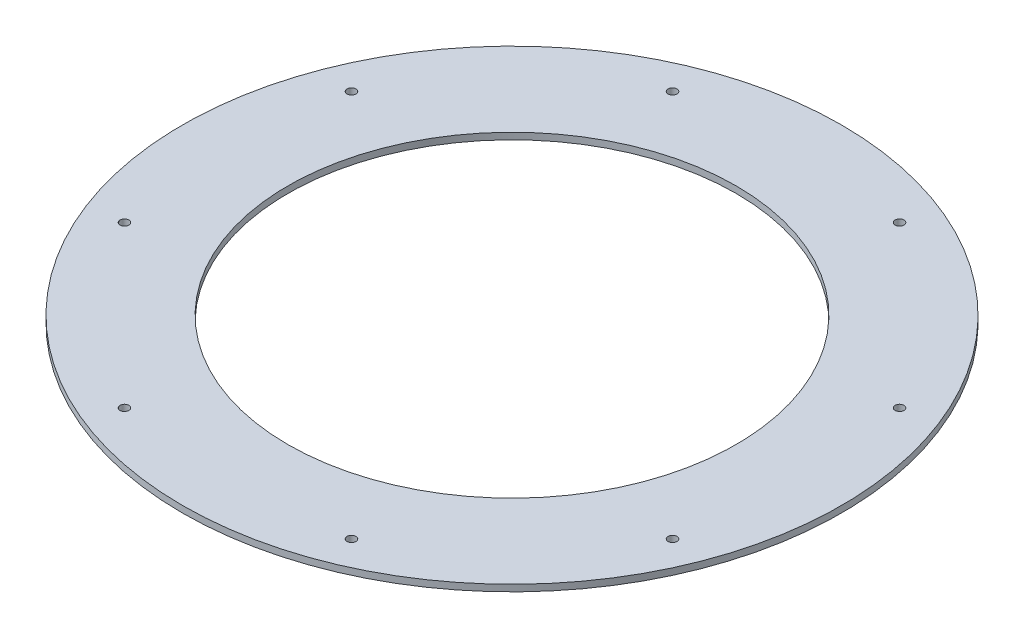
from build123d import *

# Parameters (mm, degrees)
SKETCH1_R                    = 500
SKETCH1_R_2                  = 340
BOSS_EXTRUDE1_DEPTH          = 5
F_13_5_13_5_DIAMETER_HOLE1_D = 13.5


with BuildPart() as part:
    # Sketch1 → Boss-Extrude1 (new, symmetric)
    with BuildSketch(Plane(origin=(0, 0, 0), x_dir=(1, 0, 0), z_dir=(0, 1, 0))):
        with Locations(Location((0, 0, 0), (0, 0, 270))):
            Circle(SKETCH1_R)
        with Locations(Location((0, 0, 0), (0, 0, 270))):
            Circle(SKETCH1_R_2, mode=Mode.SUBTRACT)
    extrude(amount=BOSS_EXTRUDE1_DEPTH, both=True)

    # Ø13.5 (13.5) Diameter Hole1 (through all)
    with Locations(Plane(origin=(0, 5, 0), x_dir=(1, 0, 0), z_dir=(0, 1, 0))):
        with Locations((172.207544564, 415.74578963), (415.74578963, 172.207544564), (415.74578963, -172.207544564), (172.207544564, -415.74578963), (-172.207544564, -415.74578963), (-415.74578963, -172.207544564), (-415.74578963, 172.207544564), (-172.207544564, 415.74578963)):
            Hole(F_13_5_13_5_DIAMETER_HOLE1_D / 2)


solid = part.part
